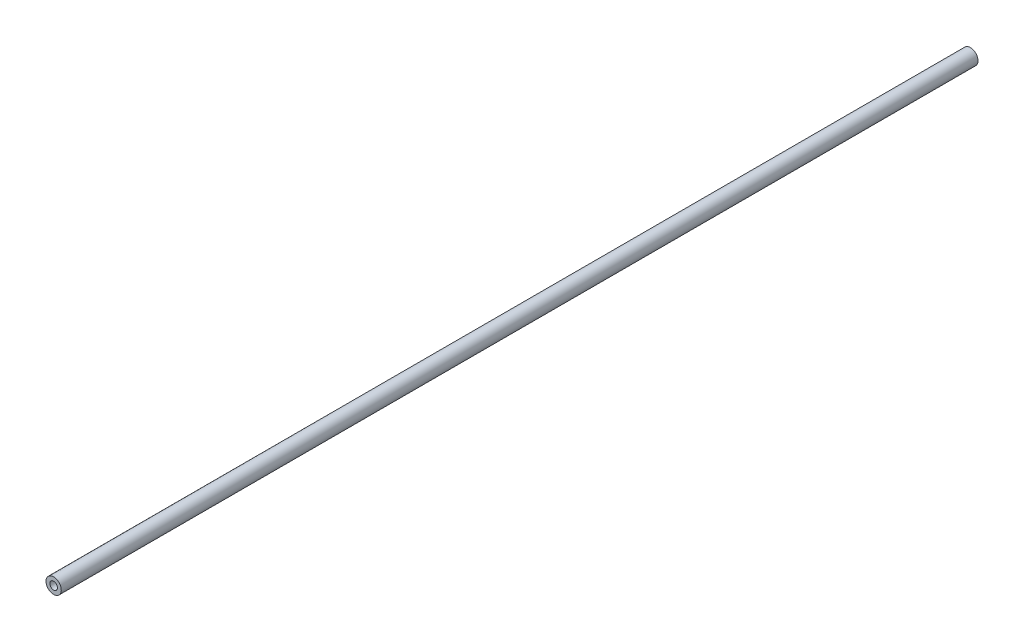
from build123d import *

# Parameters (mm, degrees)
SKETCH2_R           = 2.5
SKETCH2_R_2         = 1.25
BOSS_EXTRUDE1_DEPTH = 300


with BuildPart() as part:
    # Sketch2 → Boss-Extrude1 (new body)
    with BuildSketch(Plane.XY):
        Circle(SKETCH2_R)
        Circle(SKETCH2_R_2, mode=Mode.SUBTRACT)
    extrude(amount=BOSS_EXTRUDE1_DEPTH)


solid = part.part
